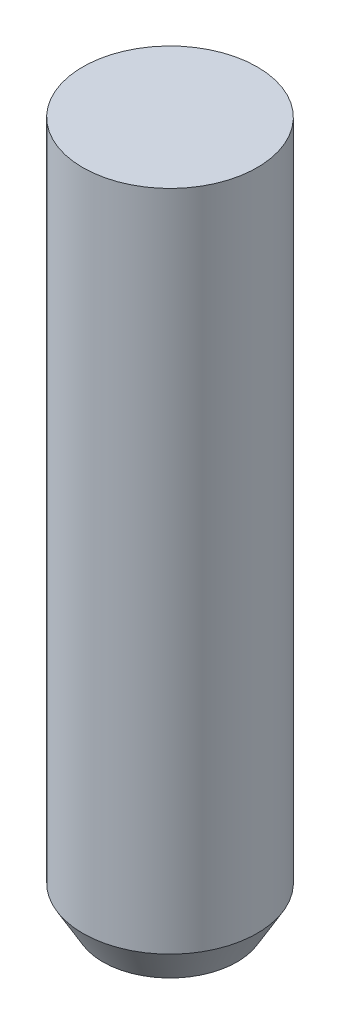
from build123d import *

# Parameters (mm, degrees)
SKETCH1_R           = 5
BOSS_EXTRUDE1_DEPTH = 40
CHAMFER1_SIZE       = 1.154700538
CHAMFER1_SIZE2      = 2


with BuildPart() as part:
    # Sketch1 → Boss-Extrude1 (new body)
    with BuildSketch(Plane(origin=(0, 0, 0), x_dir=(1, 0, 0), z_dir=(0, 1, 0))):
        with Locations(Location((0, 0, 0), (0, 0, 270))):
            Circle(SKETCH1_R)
    extrude(amount=BOSS_EXTRUDE1_DEPTH)

    # Chamfer1
    chamfer1_edges = [part.edges().sort_by_distance(p)[0] for p in [
        (0, 0, -5),
    ]]
    chamfer1_side = [part.faces().sort_by_distance(p)[0] for p in [
        (0, 0, 0),
    ]]
    chamfer(chamfer1_edges, length=CHAMFER1_SIZE, length2=CHAMFER1_SIZE2, reference=chamfer1_side[0])


solid = part.part
